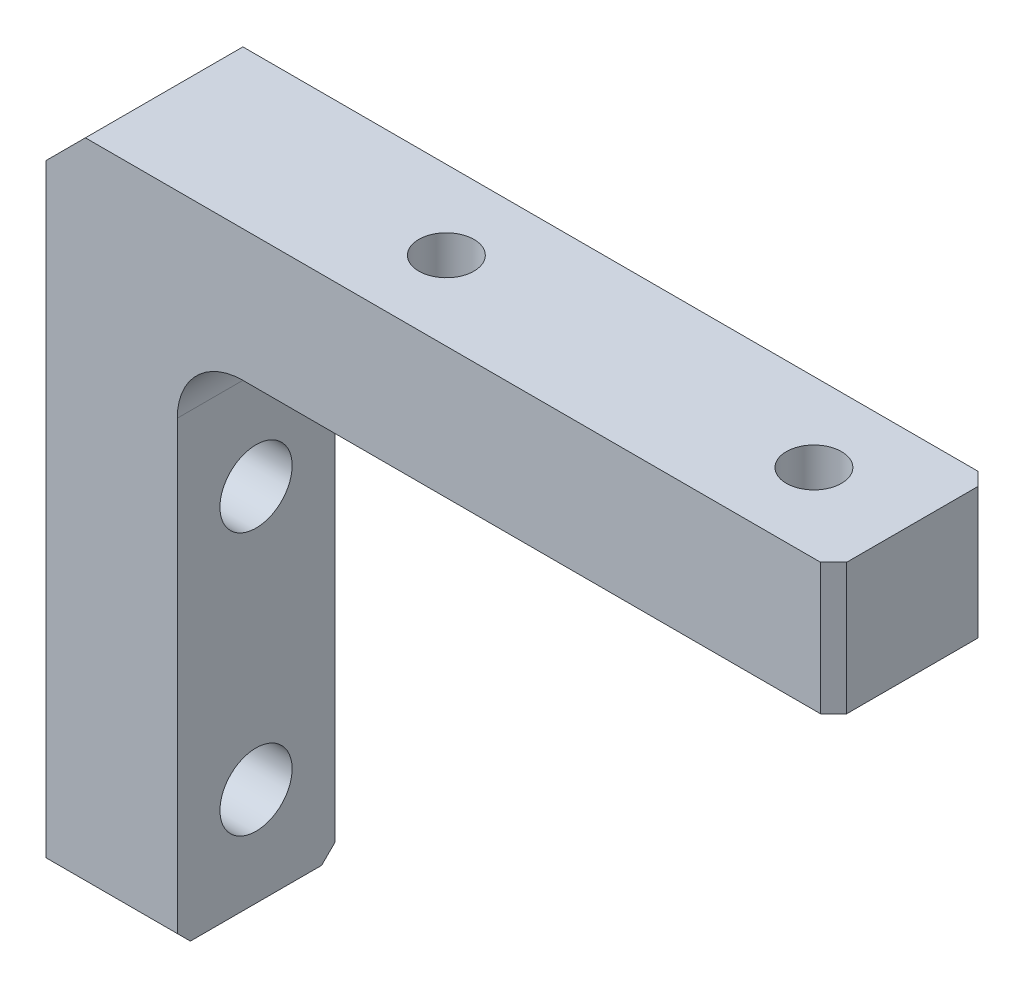
from build123d import *

# Parameters (mm, degrees)
BOSS_EXTRUDE1_DEPTH   = 12
M5_TAPPED_HOLE1_D     = 4.2
M5_TAPPED_HOLE1_DEPTH = 12.4
M5_TAPPED_HOLE1_TIP   = 1.2618073
M5_CLEARANCE_HOLE1_D  = 5.5
CHAMFER2_SIZE         = 1
FILLET1_R             = 5


with BuildPart() as part:
    # Sketch1 → Boss-Extrude1 (new body)
    with BuildSketch(Plane.XY):
        Polygon((3, 0), (60, 0), (60, -10), (10, -10), (10, -50), (0, -50), (0, -3), align=None)
    extrude(amount=BOSS_EXTRUDE1_DEPTH)

    # M5 Tapped Hole1
    with Locations(Plane(origin=(0, 0, 0), x_dir=(-1, 0, 0), z_dir=(0, 1, 0))):
        with Locations((-52.5, 6), (-24.5, 6)):
            Hole(M5_TAPPED_HOLE1_D / 2, depth=M5_TAPPED_HOLE1_DEPTH)
            with Locations((0, 0, -(M5_TAPPED_HOLE1_DEPTH + M5_TAPPED_HOLE1_TIP / 2))):  # 118° drill point
                Cone(0, M5_TAPPED_HOLE1_D / 2, M5_TAPPED_HOLE1_TIP, mode=Mode.SUBTRACT)

    # M5 Clearance Hole1 (through all)
    with Locations(Plane(origin=(10, 0, 0), x_dir=(0, 0, -1), z_dir=(1, 0, 0))):
        with Locations((-6, -42.5), (-6, -22.5)):
            Hole(M5_CLEARANCE_HOLE1_D / 2)

    # Chamfer2
    chamfer2_edges = [part.edges().sort_by_distance(p)[0] for p in [
        (60, -5, 0),
        (5, -50, 12),
        (60, -5, 12),
        (5, -50, 0),
    ]]
    chamfer(chamfer2_edges, length=CHAMFER2_SIZE)

    # Fillet1
    fillet1_edges = [part.edges().sort_by_distance(p)[0] for p in [
        (10, -10, 6),
    ]]
    fillet(fillet1_edges, radius=FILLET1_R)


solid = part.part
